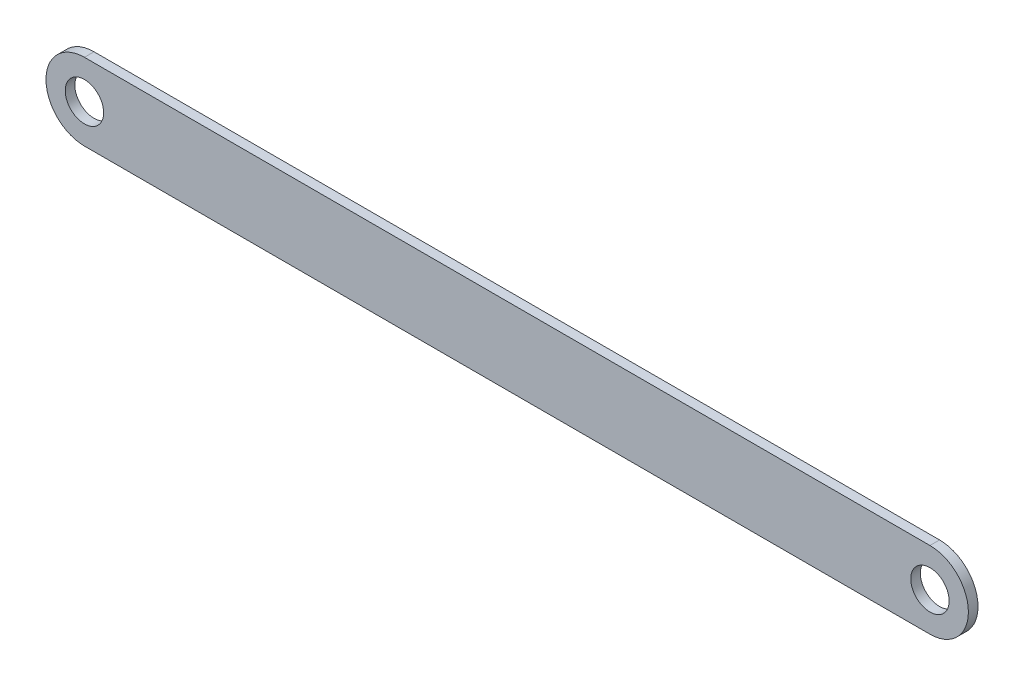
SolidWorks part; units mm, degrees
ref_plane "Front Plane" through (0, 0, 0) normal (0, 0, 1) x (1, 0, 0)
ref_plane "Top Plane" through (0, 0, 0) normal (0, 1, 0) x (1, 0, 0)
ref_plane "Right Plane" through (0, 0, 0) normal (1, 0, 0) x (0, 0, -1)
sketch "Sketch1" plane through (0, 0, 0) normal (0, 0, 1) x (1, 0, 0)
  line L0 (-110, 0) -> (110, 0) construction
  line L1 (-110, 10) -> (110, 10)
  line L2 (-110, -10) -> (110, -10)
  arc A0 (-110, 10) -> (-110, -10) centre (-110, 0) ccw
  arc A1 (110, -10) -> (110, 10) centre (110, 0) ccw
  circle A2 centre (-110, 0) radius 5
  circle A3 centre (110, 0) radius 5
  point P2 (0, 0)
  dimension "D1" = 220
  dimension "D2" = 10
  dimension "D3" = 10
extrude "Boss-Extrude1" add sketch "Sketch1" along normal blind 2.5
